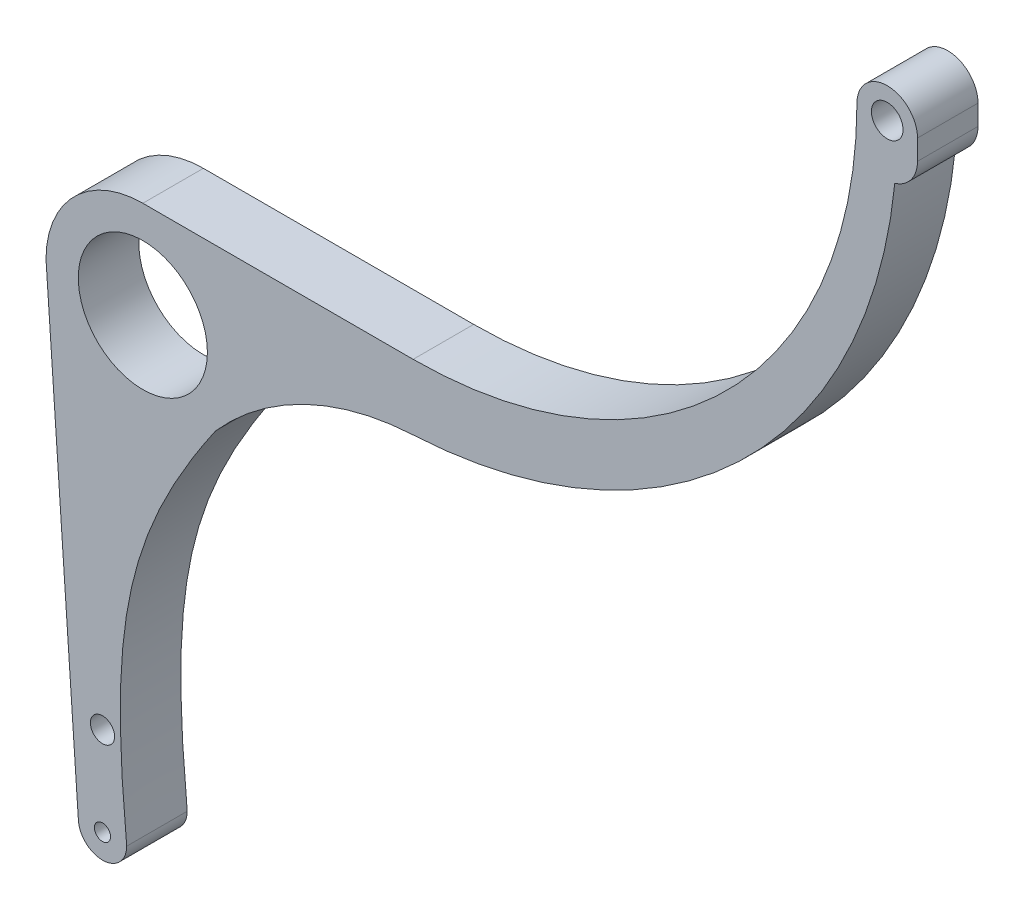
from build123d import *

# Parameters (mm, degrees)
SKETCH_1_R      = 2
SKETCH_1_R_2    = 16
SKETCH_1_R_3    = 3.91899873
SKETCH_1_R_4    = 3
EXTRUDE_3_DEPTH = 15


with BuildPart() as part:
    # 草图1 → 凸台-拉伸3 (new body)
    with BuildSketch(Plane.XY):
        with BuildLine():
            Line((-14, 116), (-6, 0))
            ThreePointArc((-6, 0), (0, -6), (6, 0))
            add(Edge.make_bspline(
                [(6, 0), (1.588652615, 45.680929706), (5.604102499, 67.643200211), (28.004797731, 100.13093391)],
                knots=[0, 0, 0, 0, 0.788155359, 0.788155359, 0.788155359, 0.788155359], degree=3))
            ThreePointArc((28.004797731, 100.13093391), (50.113637924, 116.900750568), (77, 123.767416406))
            ThreePointArc((77, 123.767416406), (157.787149523, 158.485384951), (196.379869136, 237.494896157))
            ThreePointArc((196.379869136, 237.494896157), (200.439238403, 240.311917913), (202, 245))
            Line((202, 245), (202, 250))
            ThreePointArc((202, 250), (194.5, 257.5), (187, 250))
            ThreePointArc((187, 250), (154.781745931, 172.218254069), (77, 140))
            Line((77, 140), (10, 140))
            ThreePointArc((10, 140), (-6.970562748, 132.970562748), (-14, 116))
        make_face()
        Circle(SKETCH_1_R, mode=Mode.SUBTRACT)
        with Locations((10, 116)):
            Circle(SKETCH_1_R_2, mode=Mode.SUBTRACT)
        with Locations((194.5, 250)):
            Circle(SKETCH_1_R_3, mode=Mode.SUBTRACT)
        with Locations((0, 22)):
            Circle(SKETCH_1_R_4, mode=Mode.SUBTRACT)
    extrude(amount=EXTRUDE_3_DEPTH)


solid = part.part
